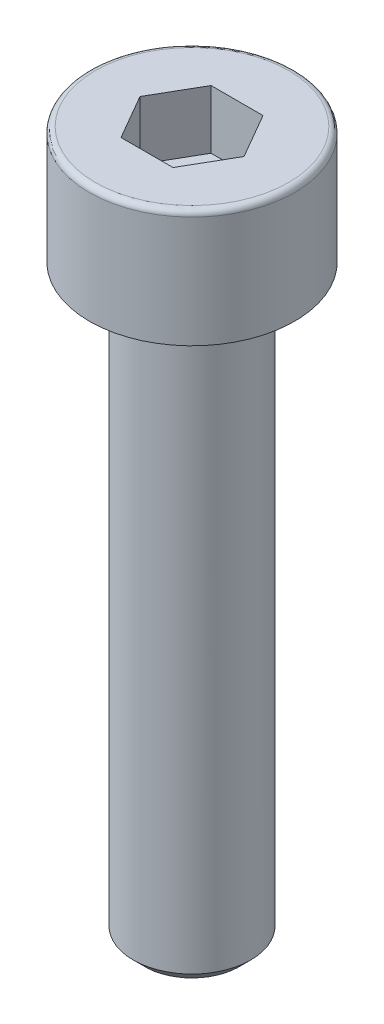
from build123d import *

# Parameters (mm, degrees)
SKETCH_1_R          = 3.5
EXTRUDE_1_DEPTH     = 4
CUT_EXTRUDE_1_DEPTH = 2
FILLET_1_R          = 0.2
SKETCH_5_R          = 2
EXTRUDE_2_DEPTH     = 20
CHAMFER_2_SIZE      = 0.39


with BuildPart() as part:
    # 草图1 → 凸台-拉伸1 (new body)
    with BuildSketch(Plane(origin=(0, 0, 0), x_dir=(1, 0, 0), z_dir=(0, 1, 0))):
        with Locations(Location((0, 0, 0), (0, 0, 270))):
            Circle(SKETCH_1_R)
    extrude(amount=EXTRUDE_1_DEPTH)

    # 草图2 → 切除-拉伸1 (cut)
    with BuildSketch(Plane(origin=(0, 4, 0), x_dir=(1, 0, 0), z_dir=(0, 1, 0))):
        Polygon((1.772465326, 0), (0.886232663, 1.535), (-0.886232663, 1.535), (-1.772465326, 0), (-0.886232663, -1.535), (0.886232663, -1.535), align=None)
    extrude(amount=-CUT_EXTRUDE_1_DEPTH, mode=Mode.SUBTRACT)

    # 圆角1
    fillet_1_edges = [part.edges().sort_by_distance(p)[0] for p in [
        (0, 4, -3.5),
    ]]
    fillet(fillet_1_edges, radius=FILLET_1_R)

    # 草图5 → 凸台-拉伸2 (add)
    with BuildSketch(Plane.XZ):
        with Locations(Location((0, 0, 0), (0, 0, 90))):
            Circle(SKETCH_5_R)
    extrude(amount=EXTRUDE_2_DEPTH)

    # 倒角2
    chamfer_2_edges = [part.edges().sort_by_distance(p)[0] for p in [
        (0, -20, -2),
    ]]
    chamfer(chamfer_2_edges, length=CHAMFER_2_SIZE)


solid = part.part
